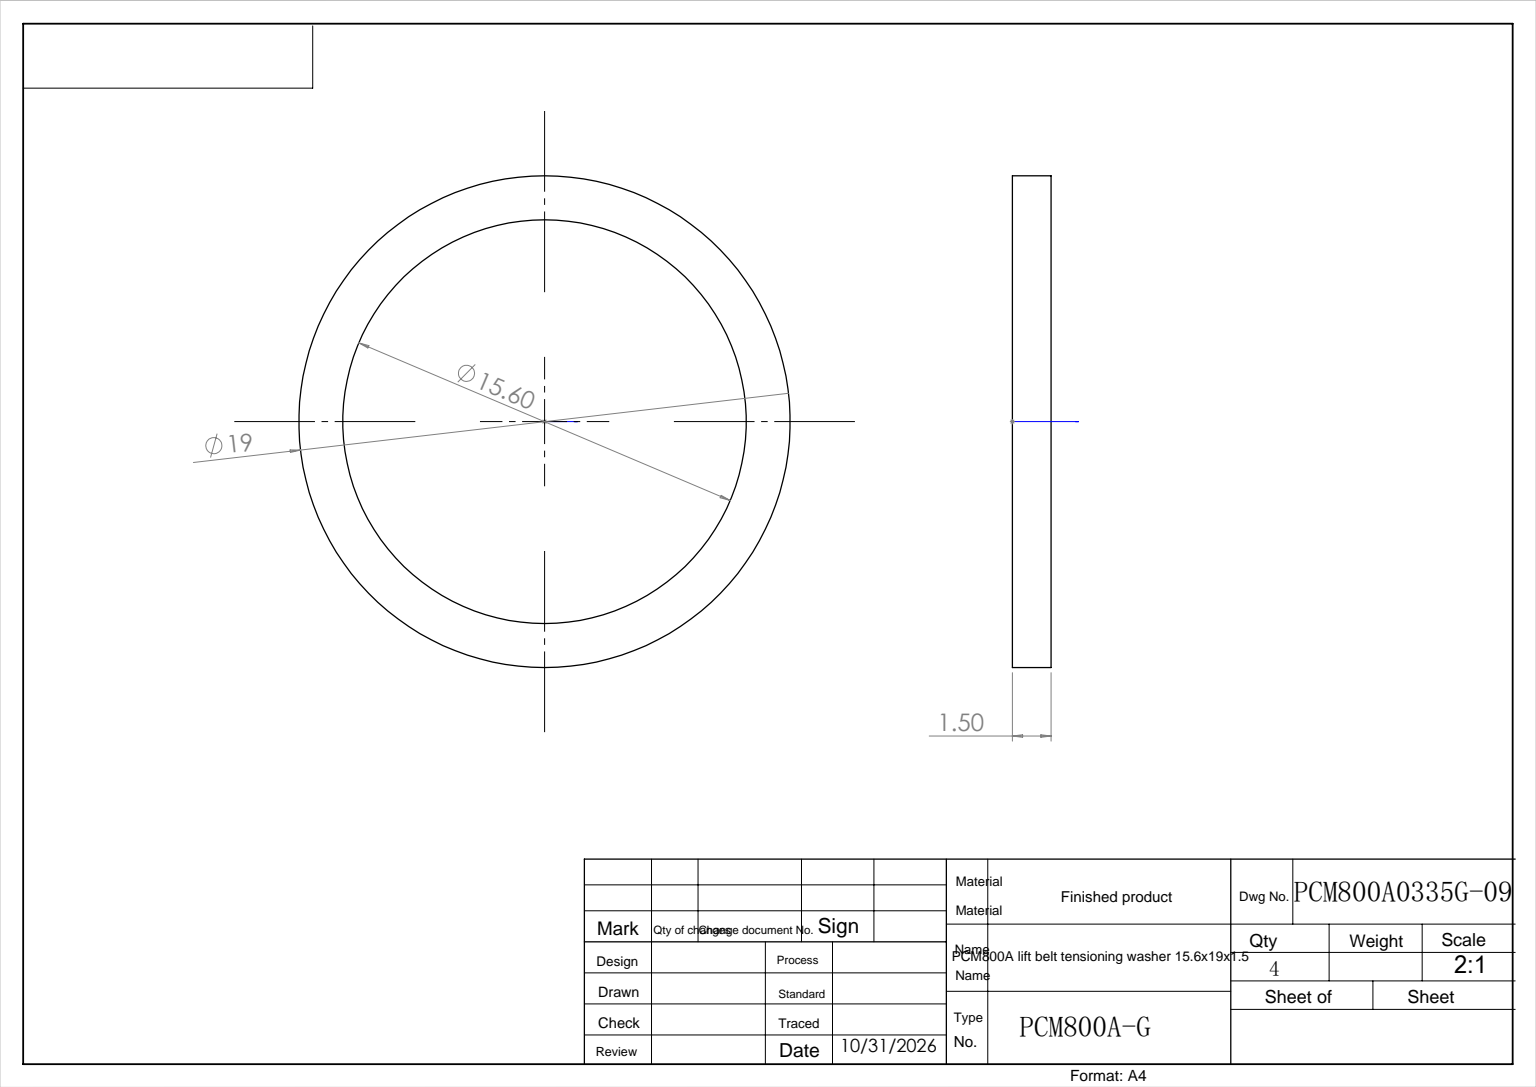
SolidWorks part; units mm, degrees
ref_plane "前视" through (0, 0, 0) normal (0, 0, 1) x (1, 0, 0)
ref_plane "上视" through (0, 0, 0) normal (0, 1, 0) x (1, 0, 0)
ref_plane "右视" through (0, 0, 0) normal (1, 0, 0) x (0, 0, -1)
sketch "草图1" plane through (0, 0, 0) normal (0, 1, 0) x (1, 0, 0)
  circle A0 centre (0, 0) radius 7.8
  circle A1 centre (0, 0) radius 9.5
extrude "拉伸1" add sketch "草图1" along normal blind 1.5
